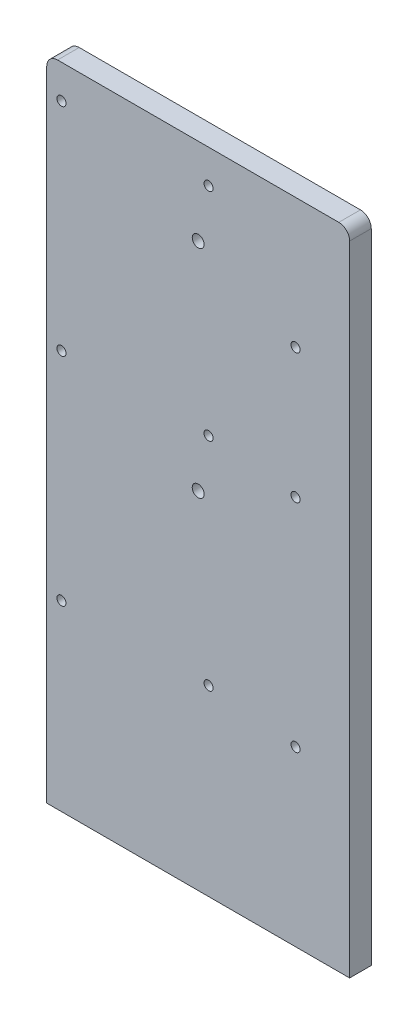
from build123d import *

# Parameters (mm, degrees)
SKETCH_1_W                = 140
SKETCH_1_H                = 300
EXTRUDE_1_DEPTH           = 10
HOLE_WIZARD_1_D           = 5.5
HOLE_WIZARD_1_DEPTH       = 14.4
HOLE_WIZARD_1_CBORE_D     = 10
HOLE_WIZARD_1_CBORE_DEPTH = 5.7
HOLE_WIZARD_1_TIP         = 1.652366702
HOLE_WIZARD_M5_1_D        = 4.2
HOLE_WIZARD_M5_2_D        = 4.2
HOLE_WIZARD_M5_2_DEPTH    = 12.4
HOLE_WIZARD_M5_2_TIP      = 1.2618073
HOLE_WIZARD_M5_3_D        = 4.2
FILLET_1_R                = 5


with BuildPart() as part:
    # 草图1 → 凸台-拉伸1 (new body)
    with BuildSketch(Plane.XY):
        Rectangle(SKETCH_1_W, SKETCH_1_H)
    extrude(amount=EXTRUDE_1_DEPTH)

    # 打孔尺寸(%根据)内六角圆柱头螺钉的类型1
    with Locations(Plane(origin=(0, 0, 0), x_dir=(-1, 0, 0), z_dir=(0, 0, -1))):
        with Locations((0, 110), (0, 10)):
            CounterBoreHole(HOLE_WIZARD_1_D / 2, HOLE_WIZARD_1_CBORE_D / 2, HOLE_WIZARD_1_CBORE_DEPTH, depth=HOLE_WIZARD_1_DEPTH)
            with Locations((0, 0, -(HOLE_WIZARD_1_DEPTH + HOLE_WIZARD_1_TIP / 2))):  # 118° drill point
                Cone(0, HOLE_WIZARD_1_D / 2, HOLE_WIZARD_1_TIP, mode=Mode.SUBTRACT)

    # M5 螺纹孔1 (through all)
    with Locations(Plane(origin=(0, 0, 0), x_dir=(-1, 0, 0), z_dir=(0, 0, -1))):
        with Locations((-4.800000353, -65.5), (63.199999647, -65.5), (-4.800000353, 34.5), (63.199999647, 34.5), (-4.800000353, 134.5), (63.199999647, 134.5)):
            Hole(HOLE_WIZARD_M5_1_D / 2)

    # M5 螺纹孔2
    with Locations(Plane(origin=(0, -150, 0), x_dir=(-1, 0, 0), z_dir=(0, -1, 0))):
        with Locations((-50, -5), (50, -5)):
            Hole(HOLE_WIZARD_M5_2_D / 2, depth=HOLE_WIZARD_M5_2_DEPTH)
            with Locations((0, 0, -(HOLE_WIZARD_M5_2_DEPTH + HOLE_WIZARD_M5_2_TIP / 2))):  # 118° drill point
                Cone(0, HOLE_WIZARD_M5_2_D / 2, HOLE_WIZARD_M5_2_TIP, mode=Mode.SUBTRACT)

    # M5 螺纹孔3 (through all)
    with Locations(Plane.XY.offset(10)):
        with Locations((45, 90), (45, 30), (45, -70)):
            Hole(HOLE_WIZARD_M5_3_D / 2)

    # 圆角1
    fillet_1_edges = [part.edges().sort_by_distance(p)[0] for p in [
        (-70, 150, 5),
        (70, 150, 5),
    ]]
    fillet(fillet_1_edges, radius=FILLET_1_R)


solid = part.part
